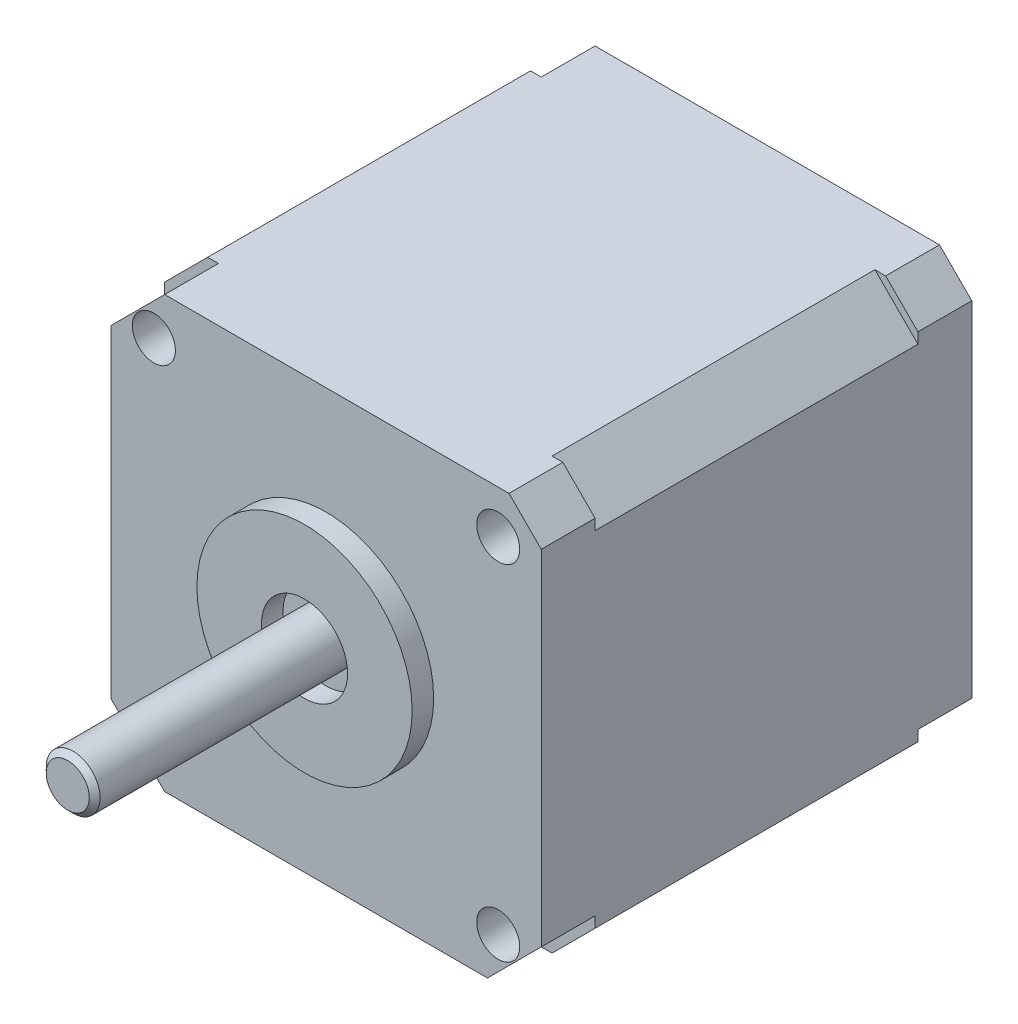
from build123d import *

# Parameters (mm, degrees)
SKETCH1_W           = 40
SKETCH1_H           = 40
BOSS_EXTRUDE1_DEPTH = 15
CHAMFER1_SIZE       = 4
BOSS_EXTRUDE2_DEPTH = 5
SKETCH4_R           = 10
BOSS_EXTRUDE3_DEPTH = 2
SKETCH5_R           = 2.5
BOSS_EXTRUDE4_DEPTH = 22
CUT_EXTRUDE1_START  = -2
SKETCH6_R           = 4
SKETCH6_R_2         = 2.5
CUT_EXTRUDE1_DEPTH  = 2
CHAMFER2_SIZE       = 0.5
SKETCH7_R           = 2
CUT_EXTRUDE2_DEPTH  = 49.989794856


with BuildPart() as part:
    # Sketch1 → Boss-Extrude1 (new, symmetric)
    with BuildSketch(Plane.XY):
        Rectangle(SKETCH1_W, SKETCH1_H)
    extrude(amount=BOSS_EXTRUDE1_DEPTH, both=True)

    # Chamfer1
    chamfer1_edges = [part.edges().sort_by_distance(p)[0] for p in [
        (-20, 20, 0),
        (20, 20, 0),
        (20, -20, 0),
        (-20, -20, 0),
    ]]
    chamfer(chamfer1_edges, length=CHAMFER1_SIZE)

    # Sketch3 → Boss-Extrude2 (add)
    with BuildSketch(Plane.XY.offset(15)):
        Polygon((15, -20), (-15, -20), (-20, -15), (-20, 15), (-15, 20), (17, 20), (20, 17), (20, -15), align=None)
    boss_extrude2 = extrude(amount=BOSS_EXTRUDE2_DEPTH)

    # Mirror1: Boss-Extrude2 across plane
    add(boss_extrude2.mirror(Plane.XY))

    # Sketch4 → Boss-Extrude3 (add)
    with BuildSketch(Plane.XY.offset(20)):
        with Locations(Location((0, 0, 0), (0, 0, 180))):
            Circle(SKETCH4_R)
    extrude(amount=BOSS_EXTRUDE3_DEPTH)

    # Sketch5 → Boss-Extrude4 (add)
    with BuildSketch(Plane.XY.offset(22)):
        Circle(SKETCH5_R)
    extrude(amount=BOSS_EXTRUDE4_DEPTH)

    # Sketch6 → Cut-Extrude1 (cut)
    with BuildSketch(Plane.XY.offset(22).offset(CUT_EXTRUDE1_START)):
        Circle(SKETCH6_R)
        Circle(SKETCH6_R_2, mode=Mode.SUBTRACT)
    extrude(amount=CUT_EXTRUDE1_DEPTH, mode=Mode.SUBTRACT)

    # Chamfer2
    chamfer2_edges = [part.edges().sort_by_distance(p)[0] for p in [
        (-2.5, 0, 44),
    ]]
    chamfer(chamfer2_edges, length=CHAMFER2_SIZE)

    # Sketch7 → Cut-Extrude2 (cut, through all)
    with BuildSketch(Plane.XY.offset(20)):
        with Locations((16, 16)):
            Circle(SKETCH7_R)
        with Locations((16, -16)):
            Circle(SKETCH7_R)
        with Locations((-16, -16)):
            Circle(SKETCH7_R)
        with Locations((-16, 16)):
            Circle(SKETCH7_R)
    extrude(amount=-CUT_EXTRUDE2_DEPTH, mode=Mode.SUBTRACT)


solid = part.part
